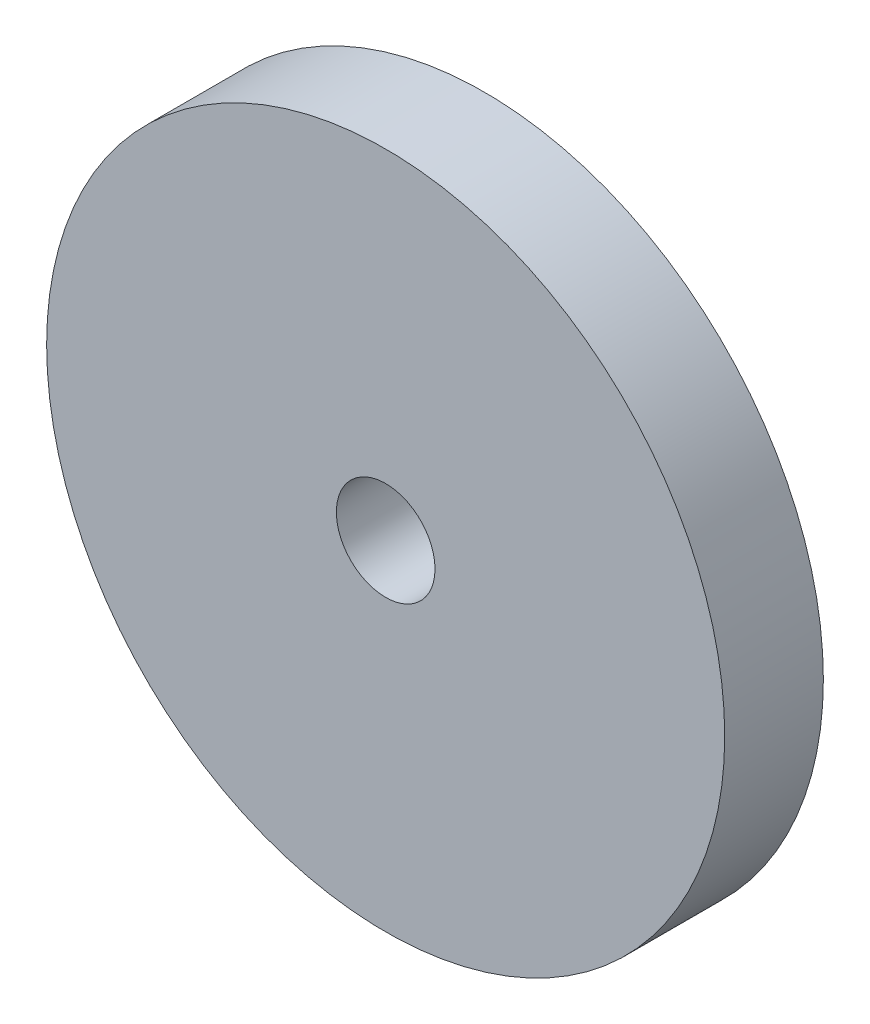
from build123d import *

# Parameters (mm, degrees)
SKETCH1_R           = 41.25
SKETCH1_R_2         = 6
BOSS_EXTRUDE1_DEPTH = 12


with BuildPart() as part:
    # Sketch1 → Boss-Extrude1 (new body)
    with BuildSketch(Plane.XY):
        Circle(SKETCH1_R)
        Circle(SKETCH1_R_2, mode=Mode.SUBTRACT)
    extrude(amount=BOSS_EXTRUDE1_DEPTH)


solid = part.part
